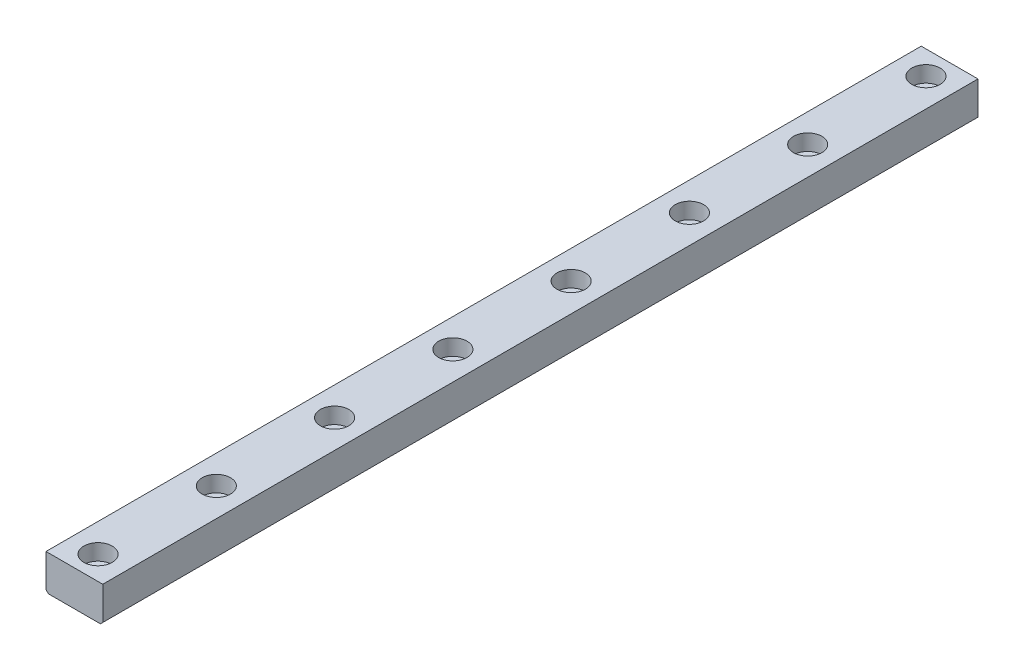
SolidWorks part; units mm, degrees
ref_plane "Front Plane" through (0, 0, 0) normal (0, 0, 1) x (1, 0, 0)
ref_plane "Top Plane" through (0, 0, 0) normal (0, 1, 0) x (1, 0, 0)
ref_plane "Right Plane" through (0, 0, 0) normal (1, 0, 0) x (0, 0, -1)
sketch "Sketch1" plane through (0, 0, 0) normal (0, 0, 1) x (1, 0, 0)
  line L1 (-6, 3.75) -> (6, 3.75)
  line L2 (-6, 3.75) -> (-6, -3.75)
  line L3 (-6, -3.75) -> (6, -3.75)
  line L4 (6, 3.75) -> (6, -3.75)
  line L5 (-6, 3.75) -> (6, -3.75) construction
  line L6 (-6, -3.75) -> (6, 3.75) construction
  point P0 (0, 0)
  dimension "D1" = 12
  dimension "D2" = 7.5
extrude "Boss-Extrude1" add sketch "Sketch1" along normal blind 185
chamfer "Chamfer1" distance 0.5 angle 45 2 edges at (6, -3.75, 92.5) (-6, -3.75, 92.5)
hole_wizard "Hole size per socket head cap screw type1" positions "Sketch3" profile "Sketch2" counterbore size "M3" standard "GB" end condition through all
sketch "Sketch3" plane through (0, 3.75, 0) normal (0, 1, 0) x (-1, 0, 0)
  line L0 (0, 0) -> (0, 185) construction
  line L1 (-6, 0) -> (6, 0) construction
  line L2 (-6, 185) -> (6, 185) construction
  point P0 (0, 5)
  dimension "D1" = 5
sketch "Sketch2" plane through (0, 3.75, 5) normal (1, 0, 0) x (0, 0, 1)
  line L0 (0, 0) -> (0, 7.5)
  line L1 (0, 7.5) -> (1.7, 7.5)
  line L3 (1.7, 7.5) -> (1.7, 3.4)
  line L4 (1.7, 3.4) -> (3, 3.4)
  line L5 (3, 3.4) -> (3, 0)
  line L7 (3, 0) -> (0, 0)
  line L11 (0, -6.35) -> (0, 107.95) construction
  dimension "通孔孔直径" = 3.4
  dimension "通孔孔深度" = 7.5
  dimension "柱形沉头孔直径" = 6
  dimension "柱形沉头孔深度" = 3.4
pattern_linear "LPattern1" count 8 spacing 25 along (0, 0, 1) of "Hole size per socket head cap screw type1"
